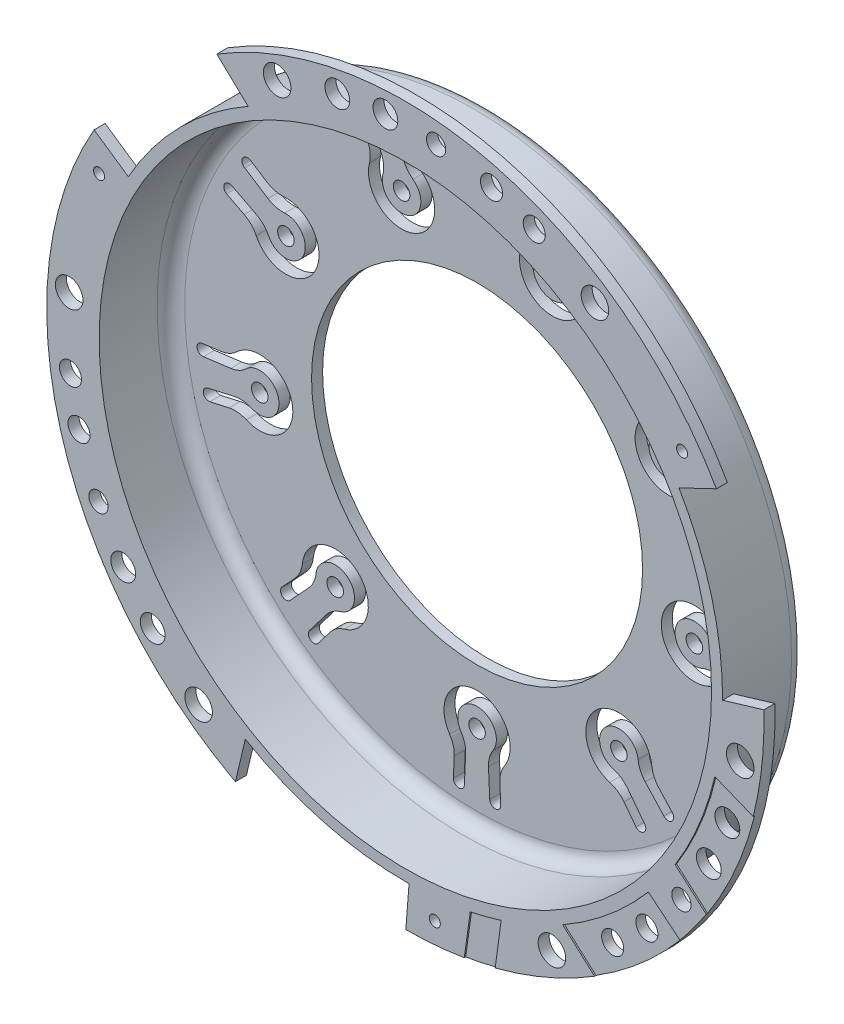
from build123d import *

# Parameters (mm, degrees)
SKETCH1_R           = 115
BOSS_EXTRUDE1_DEPTH = 30
SHELL1_T            = -4
FILLET1_R           = 5
FILLET2_R           = 5
BOSS_EXTRUDE2_START = -4
SKETCH2_R           = 130
SKETCH2_R_2         = 115
BOSS_EXTRUDE2_DEPTH = 4
SKETCH3_R           = 60
CUT_EXTRUDE1_DEPTH  = 186.677139142
SKETCH4_R           = 3
CUT_EXTRUDE2_DEPTH  = 186.677139142
SKETCH5_R           = 147.9633021
SKETCH5_R_2         = 115
CUT_EXTRUDE3_DEPTH  = 187.279360102
SKETCH6_R           = 2
SKETCH6_R_2         = 5
SKETCH6_R_3         = 4
SKETCH6_R_4         = 3.5
SKETCH6_R_5         = 4.5
BOSS_EXTRUDE3_DEPTH = 4
CUT_EXTRUDE4_DEPTH  = 0.5
SKETCH9_R           = 3.5
SKETCH9_R_2         = 5
SKETCH9_R_3         = 4.5
SKETCH9_R_4         = 4
SKETCH9_R_5         = 2
BOSS_EXTRUDE4_DEPTH = 4


with BuildPart() as part:
    # Sketch1 → Boss-Extrude1 (new body)
    with BuildSketch(Plane.XY):
        Circle(SKETCH1_R)
    extrude(amount=BOSS_EXTRUDE1_DEPTH)

    # Shell1
    shell1_openings = [part.faces().sort_by_distance(p)[0] for p in [
        (0, 0, 30),
    ]]
    offset(amount=SHELL1_T, openings=shell1_openings, kind=Kind.INTERSECTION)

    # Fillet1
    fillet1_edges = [part.edges().sort_by_distance(p)[0] for p in [
        (-115, 0, 0),
    ]]
    fillet(fillet1_edges, radius=FILLET1_R)

    # Fillet2
    fillet2_edges = [part.edges().sort_by_distance(p)[0] for p in [
        (-111, 0, 4),
    ]]
    fillet(fillet2_edges, radius=FILLET2_R)

    # Sketch2 → Boss-Extrude2 (add)
    with BuildSketch(Plane.XY.offset(30).offset(BOSS_EXTRUDE2_START)):
        Circle(SKETCH2_R)
        Circle(SKETCH2_R_2, mode=Mode.SUBTRACT)
    extrude(amount=BOSS_EXTRUDE2_DEPTH)

    # Sketch3 → Cut-Extrude1 (cut, through all)
    with BuildSketch(Plane.XY.offset(4)):
        Circle(SKETCH3_R)
    extrude(amount=-CUT_EXTRUDE1_DEPTH, mode=Mode.SUBTRACT)

    # Sketch4 → Cut-Extrude2 (cut, through all)
    with BuildSketch(Plane.XY.offset(4)):
        with Locations((0, -80)):
            Circle(SKETCH4_R)
        with Locations((-51.423008775, -61.28355545)):
            Circle(SKETCH4_R)
        with Locations((-78.784620241, -13.891854213)):
            Circle(SKETCH4_R)
        with Locations((-69.282032303, 40)):
            Circle(SKETCH4_R)
        with Locations((-27.361611466, 75.175409663)):
            Circle(SKETCH4_R)
        with Locations((27.361611466, 75.175409663)):
            Circle(SKETCH4_R)
        with Locations((69.282032303, 40)):
            Circle(SKETCH4_R)
        with Locations((78.784620241, -13.891854213)):
            Circle(SKETCH4_R)
        with Locations((51.423008775, -61.28355545)):
            Circle(SKETCH4_R)
        with BuildLine():
            Line((4.592849333, -99.894472995), (4.134289171, -89.920789471))
            ThreePointArc((4.134289171, -89.920789471), (4.491776075, -86.77350548), (5.815656194, -83.895913633))
            ThreePointArc((5.815656194, -83.895913633), (0, -73), (-5.815656194, -83.895913633))
            ThreePointArc((-5.815656194, -83.895913633), (-4.491776075, -86.77350548), (-4.134289171, -89.920789471))
            Line((-4.134289171, -89.920789471), (-4.592849333, -99.894472995))
            ThreePointArc((-4.592849333, -99.894472995), (-6.592849333, -101.894474344), (-8.592849333, -99.894472995))
            Line((-8.592849333, -99.894472995), (-8.267321685, -92.734886191))
            ThreePointArc((-8.267321685, -92.734886191), (-8.627115088, -89.57935093), (-9.958237628, -86.695782504))
            ThreePointArc((-9.958237628, -86.695782504), (0, -68), (9.958237628, -86.695782504))
            ThreePointArc((9.958237628, -86.695782504), (8.627115088, -89.57935093), (8.267321685, -92.734886191))
            Line((8.267321685, -92.734886191), (8.592849333, -99.894472995))
            ThreePointArc((8.592849333, -99.894472995), (6.592849333, -101.894472995), (4.592849333, -99.894472995))
        make_face()
        with BuildLine():
            Line((-60.692602808, -79.475832581), (-54.632920079, -71.540790949))
            ThreePointArc((-54.632920079, -71.540790949), (-52.33603407, -69.359619689), (-49.472202676, -68.006230183))
            ThreePointArc((-49.472202676, -68.006230183), (-46.923495507, -55.921244348), (-58.382304897, -60.529766695))
            ThreePointArc((-58.382304897, -60.529766695), (-59.217834273, -63.585103676), (-60.967018571, -66.225851241))
            Line((-60.967018571, -66.225851241), (-67.729256227, -73.571379292))
            ThreePointArc((-67.729256227, -73.571379292), (-70.5469212, -73.817893992), (-70.793434, -71.000228853))
            Line((-70.793434, -71.000228853), (-65.941971666, -65.724912306))
            ThreePointArc((-65.941971666, -65.724912306), (-64.189250435, -63.076361312), (-63.355427404, -60.011790668))
            ThreePointArc((-63.355427404, -60.011790668), (-43.709557459, -52.091022132), (-48.098522208, -72.813854191))
            ThreePointArc((-48.098522208, -72.813854191), (-50.971743288, -74.167166684), (-53.275699993, -76.353176195))
            Line((-53.275699993, -76.353176195), (-57.628425035, -82.04698302))
            ThreePointArc((-57.628425035, -82.04698302), (-60.446089141, -82.293496686), (-60.692602808, -79.475832581))
        make_face()
        with BuildLine():
            Line((-97.579311572, -21.869566826), (-87.836778847, -19.686061255))
            ThreePointArc((-87.836778847, -19.686061255), (-84.675232223, -19.491597), (-81.611468092, -20.295675825))
            ThreePointArc((-81.611468092, -20.295675825), (-71.89096597, -12.67631697), (-83.631224292, -8.841069208))
            ThreePointArc((-83.631224292, -8.841069208), (-86.235209682, -10.644525193), (-89.272602408, -11.543101197))
            Line((-89.272602408, -11.543101197), (-99.174391406, -12.823419563))
            ThreePointArc((-99.174391406, -12.823419563), (-101.491304595, -11.201100646), (-99.868984116, -8.884188551))
            Line((-99.868984116, -8.884188551), (-92.761640241, -7.961521501))
            ThreePointArc((-92.761640241, -7.961521501), (-89.716522119, -7.059241221), (-87.107908581, -5.247615021))
            ThreePointArc((-87.107908581, -5.247615021), (-66.966927205, -11.808076081), (-83.649448947, -24.861514266))
            ThreePointArc((-83.649448947, -24.861514266), (-86.720356492, -24.05134087), (-89.890429551, -24.244966485))
            Line((-89.890429551, -24.244966485), (-96.884718861, -25.808797838))
            ThreePointArc((-96.884718861, -25.808797838), (-99.201630723, -24.186478688), (-97.579311572, -21.869566826))
        make_face()
        with BuildLine():
            Line((-88.807575978, 45.969712299), (-79.940832595, 41.379995287))
            ThreePointArc((-79.940832595, 41.379995287), (-77.393948158, 39.496760551), (-75.563820577, 36.911450813))
            ThreePointArc((-75.563820577, 36.911450813), (-63.219854476, 36.5), (-69.748164383, 46.98446282))
            ThreePointArc((-69.748164383, 46.98446282), (-72.902172083, 47.276744929), (-75.806543424, 48.540794184))
            Line((-75.806543424, 48.540794184), (-84.214726645, 53.924760696))
            ThreePointArc((-84.214726645, 53.924760696), (-84.946778621, 56.656812178), (-82.214726645, 57.388862311))
            Line((-82.214726645, 57.388862311), (-76.177106416, 53.527153696))
            ThreePointArc((-76.177106416, 53.527153696), (-73.264436016, 52.260976292), (-70.101631236, 51.971978015))
            ThreePointArc((-70.101631236, 51.971978015), (-58.889727457, 34), (-80.059868864, 34.72380449))
            ThreePointArc((-80.059868864, 34.72380449), (-81.891551104, 37.318374637), (-84.444428101, 39.207732495))
            Line((-84.444428101, 39.207732495), (-90.807575978, 42.505610684))
            ThreePointArc((-90.807575978, 42.505610684), (-91.539626786, 45.237661492), (-88.807575978, 45.969712299))
        make_face()
        with BuildLine():
            Line((-38.481788598, 92.299252144), (-34.639682329, 83.083892146))
            ThreePointArc((-34.639682329, 83.083892146), (-33.899175613, 80.004144882), (-34.159021616, 76.84729939))
            ThreePointArc((-34.159021616, 76.84729939), (-24.967470463, 68.597561317), (-23.229163195, 80.82544252))
            ThreePointArc((-23.229163195, 80.82544252), (-25.457397949, 83.076700676), (-26.869760276, 85.911912496))
            Line((-26.869760276, 85.911912496), (-29.850055345, 95.440946118))
            ThreePointArc((-29.850055345, 95.440946118), (-28.654710851, 98.004372914), (-26.091284861, 96.809026691))
            Line((-26.091284861, 96.809026691), (-23.948457886, 89.969878791))
            ThreePointArc((-23.948457886, 89.969878791), (-22.531106057, 87.127702182), (-20.294021543, 84.873304933))
            ThreePointArc((-20.294021543, 84.873304933), (-23.257369746, 63.899098213), (-39.009386373, 78.061469212))
            ThreePointArc((-39.009386373, 78.061469212), (-38.744778831, 81.226407905), (-39.485940247, 84.314697696))
            Line((-39.485940247, 84.314697696), (-42.240559081, 90.93117157))
            ThreePointArc((-42.240559081, 90.93117157), (-41.045214126, 93.494597099), (-38.481788598, 92.299252144))
        make_face()
        with BuildLine():
            Line((29.850055345, 95.440946118), (26.869760276, 85.911912496))
            ThreePointArc((26.869760276, 85.911912496), (25.457397949, 83.076700676), (23.229163195, 80.82544252))
            ThreePointArc((23.229163195, 80.82544252), (24.967470463, 68.597561317), (34.159021616, 76.84729939))
            ThreePointArc((34.159021616, 76.84729939), (33.899175613, 80.004144882), (34.639682329, 83.083892146))
            Line((34.639682329, 83.083892146), (38.481788598, 92.299252144))
            ThreePointArc((38.481788598, 92.299252144), (41.045214588, 93.494598366), (42.240559081, 90.93117157))
            Line((42.240559081, 90.93117157), (39.485940247, 84.314697696))
            ThreePointArc((39.485940247, 84.314697696), (38.744778831, 81.226407905), (39.009386373, 78.061469212))
            ThreePointArc((39.009386373, 78.061469212), (23.257369746, 63.899098213), (20.294021543, 84.873304933))
            ThreePointArc((20.294021543, 84.873304933), (22.531106057, 87.127702182), (23.948457886, 89.969878791))
            Line((23.948457886, 89.969878791), (26.091284861, 96.809026691))
            ThreePointArc((26.091284861, 96.809026691), (28.65471039, 98.004371646), (29.850055345, 95.440946118))
        make_face()
        with BuildLine():
            Line((84.214726645, 53.924760696), (75.806543424, 48.540794184))
            ThreePointArc((75.806543424, 48.540794184), (72.902172083, 47.276744929), (69.748164383, 46.98446282))
            ThreePointArc((69.748164383, 46.98446282), (63.219854476, 36.5), (75.563820577, 36.911450813))
            ThreePointArc((75.563820577, 36.911450813), (77.393948158, 39.496760551), (79.940832595, 41.379995287))
            Line((79.940832595, 41.379995287), (88.807575978, 45.969712299))
            ThreePointArc((88.807575978, 45.969712299), (91.539627954, 45.237662166), (90.807575978, 42.505610684))
            Line((90.807575978, 42.505610684), (84.444428101, 39.207732495))
            ThreePointArc((84.444428101, 39.207732495), (81.891551104, 37.318374637), (80.059868864, 34.72380449))
            ThreePointArc((80.059868864, 34.72380449), (58.889727457, 34), (70.101631236, 51.971978015))
            ThreePointArc((70.101631236, 51.971978015), (73.264436016, 52.260976292), (76.177106416, 53.527153696))
            Line((76.177106416, 53.527153696), (82.214726645, 57.388862311))
            ThreePointArc((82.214726645, 57.388862311), (84.946777453, 56.656811503), (84.214726645, 53.924760696))
        make_face()
        with BuildLine():
            Line((99.174391406, -12.823419563), (89.272602408, -11.543101197))
            ThreePointArc((89.272602408, -11.543101197), (86.235209682, -10.644525193), (83.631224292, -8.841069208))
            ThreePointArc((83.631224292, -8.841069208), (71.89096597, -12.67631697), (81.611468092, -20.295675825))
            ThreePointArc((81.611468092, -20.295675825), (84.675232223, -19.491597), (87.836778847, -19.686061255))
            Line((87.836778847, -19.686061255), (97.579311572, -21.869566826))
            ThreePointArc((97.579311572, -21.869566826), (99.201632051, -24.186478922), (96.884718861, -25.808797838))
            Line((96.884718861, -25.808797838), (89.890429551, -24.244966485))
            ThreePointArc((89.890429551, -24.244966485), (86.720356492, -24.05134087), (83.649448947, -24.861514266))
            ThreePointArc((83.649448947, -24.861514266), (66.966927205, -11.808076081), (87.107908581, -5.247615021))
            ThreePointArc((87.107908581, -5.247615021), (89.716522119, -7.059241221), (92.761640241, -7.961521501))
            Line((92.761640241, -7.961521501), (99.868984116, -8.884188551))
            ThreePointArc((99.868984116, -8.884188551), (101.491303267, -11.201100412), (99.174391406, -12.823419563))
        make_face()
        with BuildLine():
            Line((67.729256227, -73.571379292), (60.967018571, -66.225851241))
            ThreePointArc((60.967018571, -66.225851241), (59.217834273, -63.585103676), (58.382304897, -60.529766695))
            ThreePointArc((58.382304897, -60.529766695), (46.923495507, -55.921244348), (49.472202676, -68.006230183))
            ThreePointArc((49.472202676, -68.006230183), (52.33603407, -69.359619689), (54.632920079, -71.540790949))
            Line((54.632920079, -71.540790949), (60.692602808, -79.475832581))
            ThreePointArc((60.692602808, -79.475832581), (60.446090008, -82.29349772), (57.628425035, -82.04698302))
            Line((57.628425035, -82.04698302), (53.275699993, -76.353176195))
            ThreePointArc((53.275699993, -76.353176195), (50.971743288, -74.167166684), (48.098522208, -72.813854191))
            ThreePointArc((48.098522208, -72.813854191), (43.709557459, -52.091022132), (63.355427404, -60.011790668))
            ThreePointArc((63.355427404, -60.011790668), (64.189250435, -63.076361312), (65.941971666, -65.724912306))
            Line((65.941971666, -65.724912306), (70.793434, -71.000228853))
            ThreePointArc((70.793434, -71.000228853), (70.546920333, -73.817892959), (67.729256227, -73.571379292))
        make_face()
    extrude(amount=-CUT_EXTRUDE2_DEPTH, mode=Mode.SUBTRACT)

    # Sketch5 → Cut-Extrude3 (cut, through all)
    with BuildSketch(Plane.XY.offset(30)):
        Circle(SKETCH5_R)
        Circle(SKETCH5_R_2, mode=Mode.SUBTRACT)
    extrude(amount=-CUT_EXTRUDE3_DEPTH, mode=Mode.SUBTRACT)

    # Sketch6 → Boss-Extrude3 (add)
    with BuildSketch(Plane.XY.offset(30)):
        with BuildLine():
            ThreePointArc((114.998521092, -0.583220972), (81.584885816, -81.048790283), (1.341348002, -114.992177062))
            Line((1.341348002, -114.992177062), (0.17679904, -129.999879777))
            ThreePointArc((0.17679904, -129.999879777), (93.348517578, -90.47681618), (129.941966448, 3.883987076))
            Line((129.941966448, 3.883987076), (114.998521092, -0.583220972))
        make_face()
        with Locations((10.695075918, -122.020411833)):
            Circle(SKETCH6_R, mode=Mode.SUBTRACT)
        with Locations((53.126000565, -110.049206415)):
            Circle(SKETCH6_R_2, mode=Mode.SUBTRACT)
        with Locations((74.655360065, -97.062703985)):
            Circle(SKETCH6_R_3, mode=Mode.SUBTRACT)
        with Locations((87.05977446, -86.329959327)):
            Circle(SKETCH6_R_3, mode=Mode.SUBTRACT)
        with Locations((100.070423207, -70.655222023)):
            Circle(SKETCH6_R_4, mode=Mode.SUBTRACT)
        with Locations((109.520157932, -54.877910005)):
            Circle(SKETCH6_R_5, mode=Mode.SUBTRACT)
        with Locations((116.244702742, -38.644780816)):
            Circle(SKETCH6_R_5, mode=Mode.SUBTRACT)
        with Locations((121.392658844, -16.433878994)):
            Circle(SKETCH6_R_2, mode=Mode.SUBTRACT)
    extrude(amount=-BOSS_EXTRUDE3_DEPTH)

    # Sketch8 → Cut-Extrude4 (cut)
    with BuildSketch(Plane.XY.offset(30)):
        with BuildLine():
            Line((23.537241041, -112.739111866), (21.35651636, -128.233767819))
            ThreePointArc((21.35651636, -128.233767819), (26.988290403, -127.167732468), (32.567599672, -125.854485226))
            Line((32.567599672, -125.854485226), (34.726530952, -109.809731392))
            ThreePointArc((34.726530952, -109.809731392), (29.168683536, -111.414976377), (23.537241041, -112.739111866))
        make_face()
        with BuildLine():
            Line((57.031406894, -100.057621838), (68.604938244, -110.4235593))
            ThreePointArc((68.604938244, -110.4235593), (85.133486608, -98.246065865), (99.538814595, -83.618325677))
            Line((99.538814595, -83.618325677), (88.070389266, -74.21398517))
            ThreePointArc((88.070389266, -74.21398517), (73.69264686, -88.507078016), (57.031406894, -100.057621838))
        make_face()
        with BuildLine():
            Line((97.81803979, -60.792599484), (109.077068924, -70.726183518))
            ThreePointArc((109.077068924, -70.726183518), (119.214113569, -51.845878582), (126.111739784, -31.556759793))
            Line((126.111739784, -31.556759793), (112.206131164, -25.959452796))
            ThreePointArc((112.206131164, -25.959452796), (106.446583427, -43.968556231), (97.81803979, -60.792599484))
        make_face()
    extrude(amount=-CUT_EXTRUDE4_DEPTH, mode=Mode.SUBTRACT)

    # Sketch9 → Boss-Extrude4 (add)
    # profile 1 of 2: a face of its own
    with BuildSketch(Plane.XY.offset(30)):
        with BuildLine():
            Line((-58.004344724, -99.300030177), (-61.607351748, -114.4750375))
            ThreePointArc((-61.607351748, -114.4750375), (-124.987606803, -35.750498536), (-112.823505109, 64.582170101))
            Line((-112.823505109, 64.582170101), (-100.406084901, 56.067977623))
            ThreePointArc((-100.406084901, 56.067977623), (-110.942645162, -30.277540926), (-58.004344724, -99.300030177))
        make_face()
        with Locations((-111.224428786, -51.335917653)):
            Circle(SKETCH9_R, mode=Mode.SUBTRACT)
        with Locations((-74.928486114, -96.912186895)):
            Circle(SKETCH9_R_2, mode=Mode.SUBTRACT)
        with Locations((-102.285743137, -67.408283993)):
            Circle(SKETCH9_R_3, mode=Mode.SUBTRACT)
        with Locations((-91.589713282, -81.348475222)):
            Circle(SKETCH9_R_3, mode=Mode.SUBTRACT)
        with Locations((-121.386447443, -16.122086352)):
            Circle(SKETCH9_R_4, mode=Mode.SUBTRACT)
        with Locations((-118.293825114, -32.230996666)):
            Circle(SKETCH9_R_4, mode=Mode.SUBTRACT)
        with Locations((-121.868408704, 9.016137117)):
            Circle(SKETCH9_R_2, mode=Mode.SUBTRACT)
        with Locations((-111.020314387, 51.747998476)):
            Circle(SKETCH9_R_5, mode=Mode.SUBTRACT)
    # profile 2 of 2: a face of its own
    with BuildSketch(Plane.XY.offset(30)):
        with BuildLine():
            Line((99.19599055, 58.182088815), (112.770308085, 64.675015379))
            ThreePointArc((112.770308085, 64.675015379), (31.948447227, 126.013081542), (-68.3346147, 110.591050424))
            Line((-68.3346147, 110.591050424), (-56.994176368, 99.883251149))
            ThreePointArc((-56.994176368, 99.883251149), (29.664709927, 111.108077946), (99.19599055, 58.182088815))
        make_face()
        with Locations((100.325238468, 70.272413357)):
            Circle(SKETCH9_R_5, mode=Mode.SUBTRACT)
        with Locations((46.731087378, 113.184790337)):
            Circle(SKETCH9_R_4, mode=Mode.SUBTRACT)
        with Locations((-46.46417273, 113.346065889)):
            Circle(SKETCH9_R_2, mode=Mode.SUBTRACT)
        with Locations((-7.234414795, 122.286193998)):
            Circle(SKETCH9_R_3, mode=Mode.SUBTRACT)
        with Locations((-24.654989461, 119.993256038)):
            Circle(SKETCH9_R_3, mode=Mode.SUBTRACT)
        with Locations((11.154005579, 121.991139676)):
            Circle(SKETCH9_R, mode=Mode.SUBTRACT)
        with Locations((31.234050655, 118.560955993)):
            Circle(SKETCH9_R_4, mode=Mode.SUBTRACT)
        with Locations((68.742408139, 101.033069298)):
            Circle(SKETCH9_R_2, mode=Mode.SUBTRACT)
    extrude(amount=-BOSS_EXTRUDE4_DEPTH)


solid = part.part
